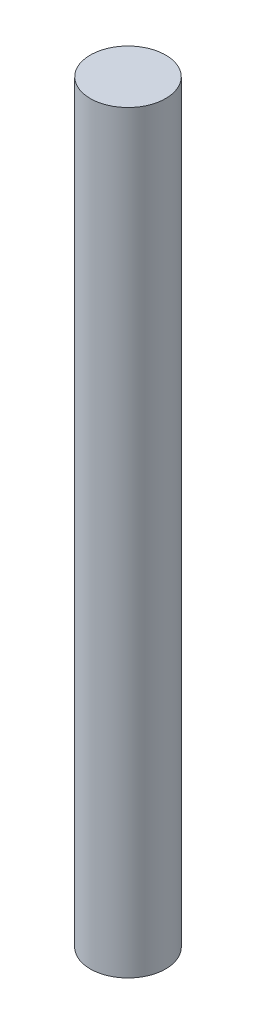
SolidWorks part; units mm, degrees
ref_plane "Front Plane" through (0, 0, 0) normal (0, 0, 1) x (1, 0, 0)
ref_plane "Top Plane" through (0, 0, 0) normal (0, 1, 0) x (1, 0, 0)
ref_plane "Right Plane" through (0, 0, 0) normal (1, 0, 0) x (0, 0, -1)
sketch "Sketch1" plane through (0, 0, 0) normal (0, 1, 0) x (1, 0, 0)
  circle A0 centre (0, 0) radius 10
  dimension "D1" = 20
extrude "Boss-Extrude1" add sketch "Sketch1" along normal blind 200
hole_wizard "M6 Tapped Hole1" positions "Sketch2" profile "Sketch3" tap size "M6" standard "GB"
sketch "Sketch2" plane through (0, 0, 0) normal (0, -1, 0) x (-1, 0, 0)
  point P0 (0, 0)
sketch "Sketch3" plane through (0, 0, 0) normal (1, 0, 0) x (0, 0, -1)
  line L0 (0, 0) -> (0, 16.5022)
  line L1 (0, 16.5022) -> (2.5, 15)
  line L2 (2.5, 15) -> (2.5, 0)
  line L5 (2.5, 0) -> (0, 0)
  line L10 (0, 16.5022) -> (-2.5, 15) construction
  line L11 (0, -6.35) -> (0, 107.95) construction
  dimension "螺纹孔钻头直径" = 5
  dimension "螺纹孔钻头深度" = 15
  dimension "导头角度" = 118
cosmetic thread "Hole Cosmetic Thread1" parameters "D1"=12, "D2"=6
